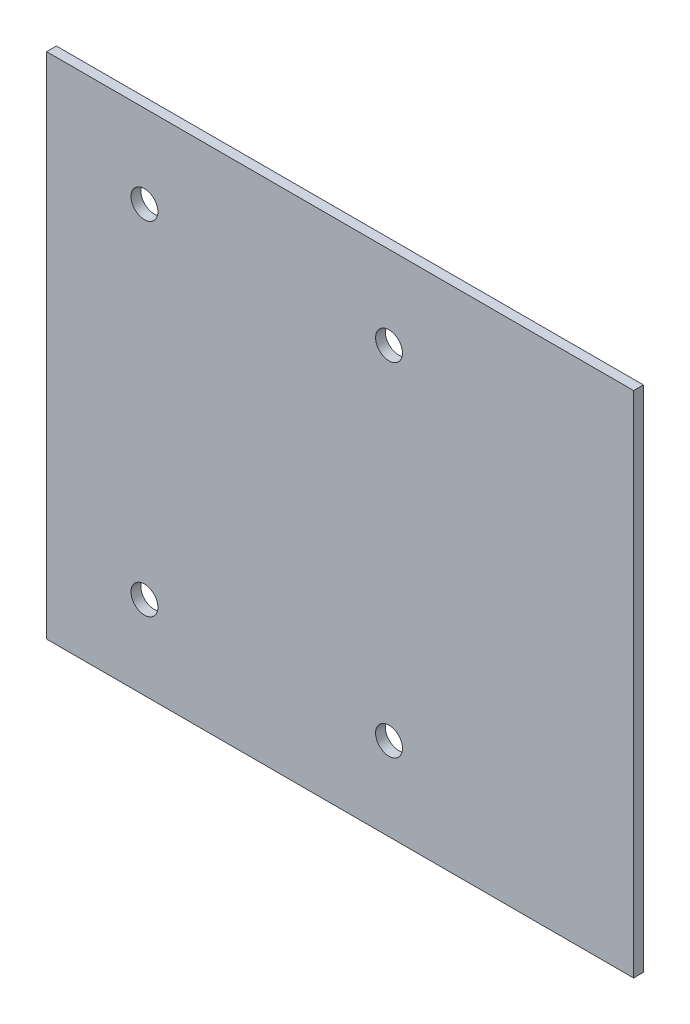
SolidWorks part; units mm, degrees
material "Q235"
ref_plane "前视基准面" through (0, 0, 0) normal (0, 0, 1) x (1, 0, 0)
ref_plane "上视基准面" through (0, 0, 0) normal (0, 1, 0) x (1, 0, 0)
ref_plane "右视基准面" through (0, 0, 0) normal (1, 0, 0) x (0, 0, -1)
sketch "草图1" plane through (0, 0, 0) normal (0, 0, 1) x (1, 0, 0)
  line L1 (120, -104) -> (-120, -104)
  line L2 (120, -104) -> (120, 104)
  line L3 (120, 104) -> (-120, 104)
  line L4 (-120, -104) -> (-120, 104)
  line L5 (120, -104) -> (-120, 104) construction
  line L6 (120, 104) -> (-120, -104) construction
  point P0 (0, 0)
  dimension "D1" = 240
  dimension "D2" = 208
extrude "凸台-拉伸1" add sketch "草图1" along normal blind 4
sketch "草图2" plane through (0, 0, 0) normal (0, 0, -1) x (-1, 0, 0)
  line L0 (146.9924, 0) -> (-176.8036, 0) construction
  line L1 (80, 70) -> (-20, 70) construction
  line L2 (80, 70) -> (80, -70) construction
  line L3 (80, -70) -> (-20, -70) construction
  line L4 (-20, 70) -> (-20, -70) construction
  line L5 (80, 70) -> (-20, -70) construction
  line L6 (80, -70) -> (-20, 70) construction
  circle A0 centre (-20, -70) radius 5.5
  circle A1 centre (80, -70) radius 5.5
  circle A2 centre (80, 70) radius 5.5
  circle A3 centre (-20, 70) radius 5.5
  point P0 (30, 0)
  dimension "D3" = 11
  dimension "D1" = 140
  dimension "D2" = 100
  dimension "D6" = 30
  dimension "D4" = 2
  dimension "D5" = 2
extrude "切除-拉伸1" cut sketch "草图2" against normal blind 10
